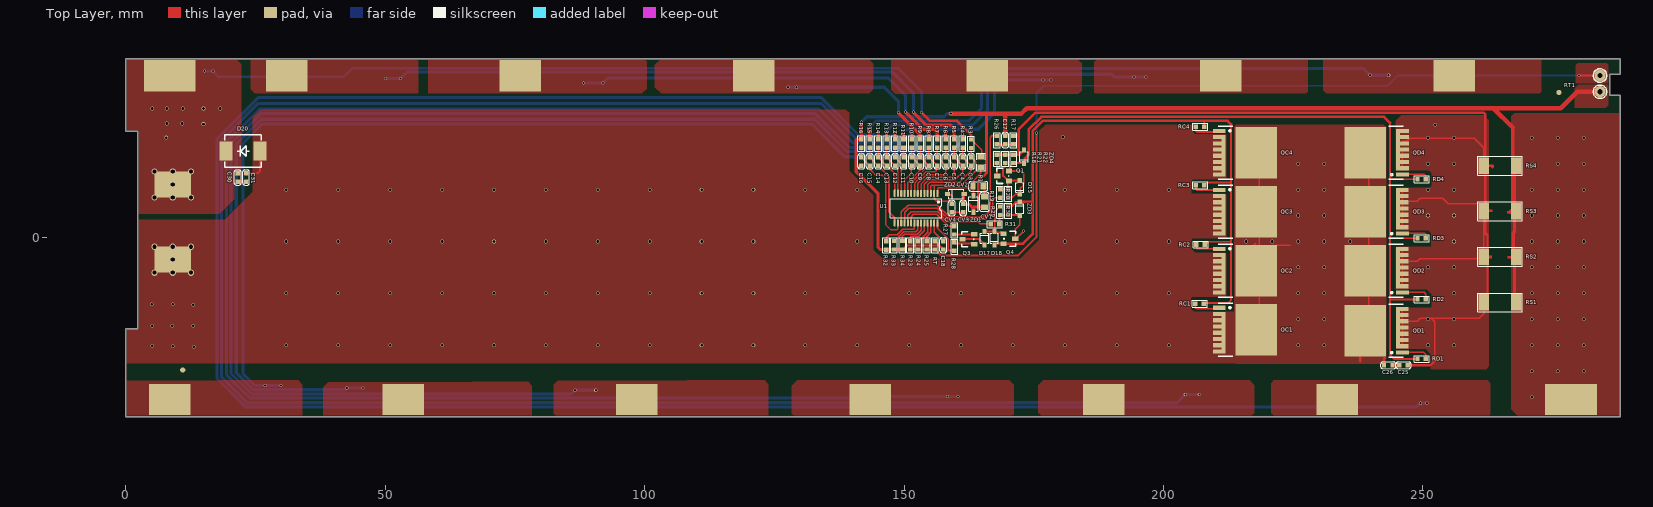
[diagram p0: Top Layer view]
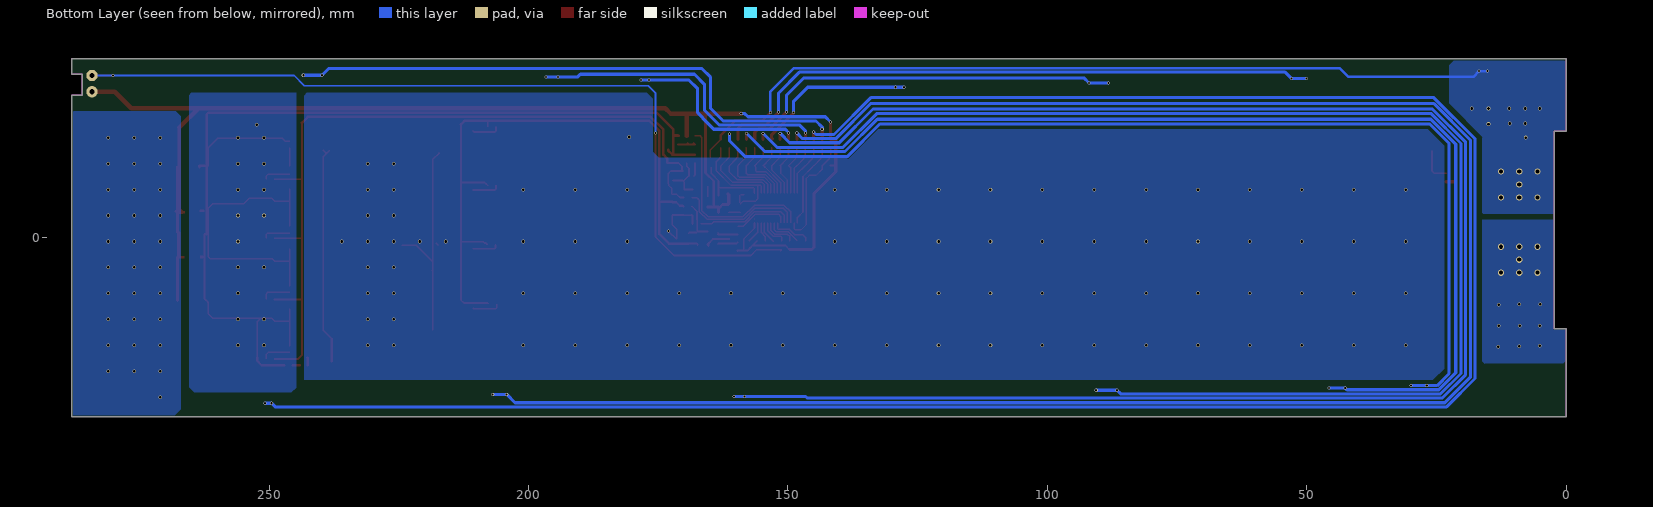
[diagram p1: Bottom Layer view, seen from below]
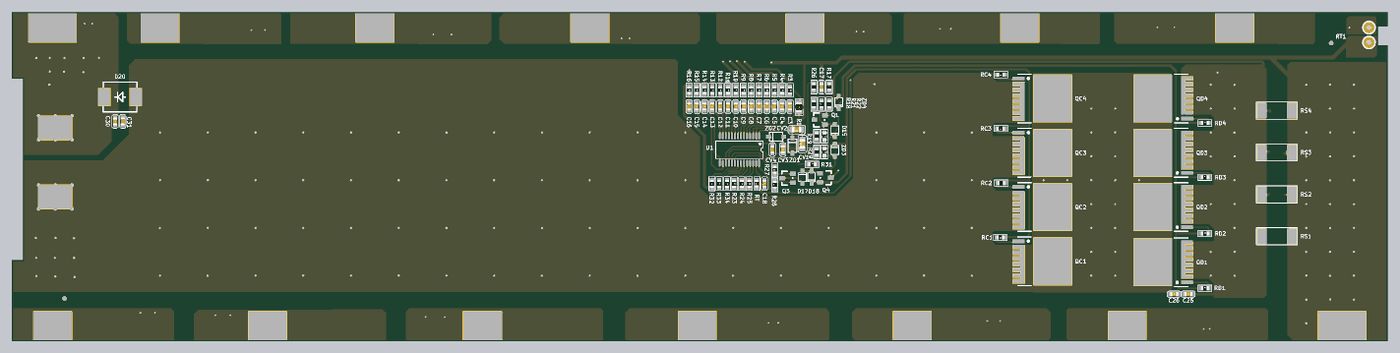
[diagram p2: 3D render of the assembled board from above, using the file's embedded part models]
# Altium PCB MISC84297.PcbDoc
Units mm, origin at the board's own origin, x right, y up, seen from the top; angles counter-clockwise.
Board outline 288 x 69 mm, 2 copper layers (Top Layer, Bottom Layer); 91 components, 64 nets, 295 pads, 210 vias.

## Layer stack, top to bottom (the 12.6 mil dielectric is the usual default, probably not edited)
Top Solder: solder mask 0.0102, Solder Resist, Dk 3.5
Top Layer: signal copper 0.0356
Dielectric 1: dielectric 0.32, FR-4, Dk 4.8
Bottom Layer: signal copper 0.0356
Bottom Solder: solder mask 0.0102, Solder Resist, Dk 3.5

## Board outline
0,-34.5 0,-17.5 2.3,-17.5 2.3,20.5 0,20.5 0,34.5 288,34.5 288,31.5 286,31.5 286,27.5 288,27.5 288,-34.5

## Design rules (kind name [scope] priority, off if disabled: settings)
Clearance [All] p1: gap=0.2 ignorepadtopadclearanceinfootprint=FALSE
ComponentClearance [All] p1: gap=0.2 collisioncheckmode=3 verticalgap=0.254 showdistances=FALSE
PolygonConnect [All] p1: connectstyle=Direct reliefconductorwidth=0.254 reliefentries=4 polygonreliefangle="90 Angle" airgapwidth=0.254
RoutingVias [All] p1: holewidth=0.4 width=0.6 viastyle="Through Hole" minholewidth=0.4 minwidth=0.6 maxholewidth=0.4 maxwidth=0.6
SolderMaskExpansion [All] p1: expansion=0.102 istentingtop=FALSE
SupplyNets "Schematic Supply Nets" [InNet('B-')] p1: voltage=0.000
Width [All] p1: maxlimit=1 minlimit=0.2 preferedwidth=0.25
29 further rules are at their usual default settings.

## Components (designator, comment, footprint, x,y, rotation, side; value= is the part's Value field where it differs from the comment)
C3 "104" CAP0603 162.922,14.7 r0 top
C4 "104" CAP0603 161.295,14.7 r0 top
C5 "104" CAP0603 159.668,14.7 r0 top
C6 "104" CAP0603 158.04,14.7 r0 top
C7 "104" CAP0603 156.413,14.7 r0 top
C8 "104" CAP0603 154.786,14.7 r0 top
C9 "104" CAP0603 153.158,14.7 r0 top
C10 "104" CAP0603 151.531,14.7 r0 top
C11 "104" CAP0603 149.904,14.7 r0 top
C12 "104" CAP0603 148.276,14.7 r0 top
C13 "104" CAP0603 146.649,14.7 r0 top
C14 "104" CAP0603 145.022,14.7 r0 top
C15 "104" CAP0603 143.395,14.7 r0 top
C16 "0.47uF" CAP0603 141.767,14.7 r0 top
C17 "104" CAP0603 169.5,18.8 r180 top
C18 "104" CAP0603 157.55,-1.467 r0 top
C25 "0.1uF" CAP0603 246.255,-24.587 r270 top
C26 "0.1uF" CAP0603 243.32,-24.587 r270 top
C30 "0.1uF" CAP0603 21.6,11.6 r180 top
C31 "0.1uF" CAP0603 23.2,11.6 r0 top
CV1 "2.2uF" CAP0805 165.5,6.9 r90 top
CV2 "2.2uF" CAP0805 164.3,9.9 r180 top
CV3 "0.1uF" CAP0603 161.4,5.7 r0 top
CV4 "0.1uF" CAP0603 159.2,5.7 r180 top
D15 "1N4148" SOD323 172.3,9.7 r270 top
D17 "1N4148" SOD323 165.5,-0.1 r90 top
D18 "1N4148" SOD323 167.4,-0.1 r270 top
D20 "RS3M" SMC 22.625,16.7 r180 top
Q1 "MMBT5401" SOT-23-3 169.1,11.9 r90 top
Q3 "MMBT5401" SOT-23-3 162.4,-0.3 r90 top
Q4 "MMBT5401" SOT-23-3 170.3,-0.2 r270 top
QC1 "NMOS" TOLL_123 214.383,-17.712 r270 top
QC2 "NMOS" TOLL_123 214.383,-6.349 r270 top
QC3 "NMOS" TOLL_123 214.383,5.021 r270 top
QC4 "NMOS" TOLL_123 214.383,16.388 r270 top
QD1 "NMOS" TOLL_123 242.393,-17.912 r90 top
QD2 "NMOS" TOLL_123 242.393,-6.349 r90 top
QD3 "NMOS" TOLL_123 242.393,5.021 r90 top
QD4 "NMOS" TOLL_123 242.422,16.388 r90 top
R1 "2K" RES0805 164.8,15.6 r270 top
R3 "2K" RES0603 162.922,18.1 r0 top
R4 "2K" RES0603 161.277,18.15 r0 top
R5 "2K" RES0603 159.651,18.15 r0 top
R6 "2K" RES0603 158.025,18.15 r0 top
R7 "2K" RES0603 156.399,18.15 r0 top
R8 "2K" RES0603 154.774,18.15 r0 top
R9 "2K" RES0603 153.148,18.15 r0 top
R10 "2K" RES0603 151.522,18.15 r0 top
R11 "2K" RES0603 149.896,18.15 r0 top
R12 "2K" RES0603 148.27,18.15 r0 top
R13 "2K" RES0603 146.645,18.15 r0 top
R14 "2K" RES0603 145.019,18.15 r0 top
R15 "2K" RES0603 143.393,18.15 r0 top
R16 "2K" RES0603 141.767,18.15 r0 top
R17 "1K" RES0603 171.1,18.8 r180 top
R18 "510R" RES0603 167.9,15.19 r180 top
R19 "1K" RES0603 168.5,8.5 r180 top
R20 "NC" RES0603 170.1,8.5 r0 top
R21 "5.1M" RES0603 169.5,15.2 r180 top
R22 "5.1M" RES0603 171.1,15.2 r180 top
R23 "270K" RES0603 151.185,-1.467 r0 top
R24 "41.2K" RES0603 152.776,-1.467 r0 top
R25 "22K" RES0603 154.367,-1.467 r0 top
R26 "10K" RES0603 167.9,18.8 r180 top
R27 "10K" RES0603 159.7,1.41 r180 top
R28 "3M" RES0603 159.7,-1.7 r180 top
R29 "5.1M" RES0603 168.5,5.2 r0 top
R30 "5.1M" RES0603 170.1,5.2 r0 top
R31 "1M" RES0603 167.51,2.6 r90 top
R32 "200K" RES0603 146.55,-1.482 r0 top
R33 "200K" RES0603 148.075,-1.457 r0 top
R34 "499K" RES0603 149.7,-1.457 r0 top
RC1 "47R" RES0603 206.955,-12.712 r270 top
RC2 "47R" RES0603 207.145,-1.312 r270 top
RC3 "47R" RES0603 207.045,10.088 r270 top
RC4 "47R" RES0603 207.055,21.388 r270 top
RD1 "47R" RES0603 249.745,-23.362 r90 top
RD2 "47R" RES0603 249.745,-11.887 r90 top
RD3 "47R" RES0603 249.745,-0.112 r90 top
RD4 "47R" RES0603 249.745,11.263 r90 top
RS1 "" 2512 264.795,-12.462 r90 top
RS2 "" 2512 264.795,-3.687 r90 top
RS3 "" 2512 264.795,5.088 r90 top
RS4 "" 2512 264.795,13.863 r90 top
RT "NC" RES0603 155.959,-1.467 r180 top
RT1 "103AT B=3435" WK 284.092,29.627 r270 top locked
U1 "CW1143" SSOP-28-0.635 152.322,5.7 r270 top locked
ZD1 "68V" SOD123 163.4,6.5 r90 top
ZD2 "68V" SOD123 160,8.4 r180 top
ZD3 "15V" SOD323 172.3,5.6 r90 top
ZD4 "15V" SOD323 173.1,15.6 r270 top

## Footprints (in the part's own frame and the unit in brackets; to place one, negate y for a bottom-side part, rotate by r counter-clockwise, add the part's x,y. Pads: shape width x height; smd on the part's side, far side on the other; paste and mask are expansions set on the pad)
2512 [mm]
  rect 3.2x2 smd: 1(0,3.05) 2(0,-3.15)
  silkscreen extent -1.8,-4.33 1.8,4.25
CAP0603 [mm] "CAP0402"
  rect 0.88x0.83 smd mask+0: 1(0,0.81) 2(0,-0.81)
  silkscreen extent -0.65,-1.45 0.65,1.45, body extent -0.41,-0.79 0.4,0.81, height 0.88
CAP0805 [mil]
  rect 43.31x50 smd: 1(-40,0)
  rect 40x50 smd: 2(40,0)
  silkscreen extent -73,-36 71,36, body extent -39,-25 39,25, height 35
RES0603 [mm] "CAP0402"
  rect 0.88x0.83 smd mask+0: 1(0,0.81) 2(0,-0.81)
  silkscreen extent -0.65,-1.45 0.65,1.45, body extent -0.4,-0.83 0.4,0.77, height 0.3
RES0805 [mil]
  rect 40x50 smd: 1(0,0) 2(80,0)
  silkscreen extent -28,-32 107,32, body extent 1,-25 79,24, height 4
SMC [mm]
  rect 2.44x3.62 smd: 1(-3.275,0) 2(3.275,0)
  silkscreen extent -3.55,-3.1 3.55,3.1
SOD123 [mm]
  rect 1x0.8 smd: 1(-1.6,0) 2(1.6,0)
  silkscreen extent -1.4,-0.9 1.4,0.9
SOD323 [mm]
  rect 1x0.8 smd: 1(-1.3,0) 2(1.3,0)
  silkscreen extent -0.92,-0.8 0.93,0.8
SOT-23-3 [mil]
  rect 36x47.24 smd: 1(-37.5,-43.94) 2(37.5,-43.94) 3(0.5,43.94)
  silkscreen extent -58,-41 58,49
SSOP-28-0.635 [mm]
  rect 1.4x0.4 smd: 1(-2.838,4.127) 28(2.862,4.128)
  oval 1.4x0.4 smd: 2(-2.838,3.492) 3(-2.838,2.857) 4(-2.838,2.222) 5(-2.838,1.587) 6(-2.838,0.952) 7(-2.838,0.317) 8(-2.838,-0.318) 9(-2.838,-0.953) 10(-2.838,-1.588) 11(-2.838,-2.223) 12(-2.838,-2.858) 13(-2.862,-3.493) 14(-2.862,-4.128) 15(2.862,-4.127) 16(2.862,-3.492) 17(2.862,-2.857) 18(2.862,-2.222) 19(2.862,-1.587) 20(2.862,-0.952) 21(2.862,-0.317) 22(2.862,0.318) 23(2.862,0.953) 24(2.862,1.588) 25(2.862,2.223) 26(2.862,2.858) 27(2.862,3.493)
  silkscreen extent -1.79,-4.96 1.86,4.96
TOLL_123 [mm] "贴片MOS"
  rect 0.8x2.5 smd: 1(-4.2,-3.638)
  rect 0.8x1.7 smd: 2(-3,-4) 2(-1.8,-4) 2(-0.6,-4) 2(0.6,-4) 2(1.8,-4) 2(3,-4) 2(4.2,-4)
  rect 8x0.8 smd: 2(0.6,-2.788)
  rect 9.9x8 smd: 3(0,3.5)
  silkscreen extent -5.1,-3.8 5.1,-1
WK [mm]
  round 2.2 hole 1: 1(-1.625,0.025) 2(1.5,0.025)
  silkscreen extent -2.91,-1.27 2.8,1.33

## Part data
C3 C4 C5 C6 C7 C8 C9 C10 C11 C12 C13 C14 C15 C16 C17 C18 C25 C26 C30 C31 CV1 CV2 CV3 CV4: library part CAP
D15 D17 D18 D20: library part DIODE, "DIODE"
Q1 Q3 Q4: library part PNP, "PNP Bipolar Transistor"
R1 R3 R4 R5 R6 R7 R8 R9 R10 R11 R12 R13 R14 R15 R16 R17 R18 R19 R20 R21 R22 R23 R24 R25 R26 R27 R28 R29 R30 R31 R32 R33 R34 RC1 RC2 RC3 RC4 RD1 RD2 RD3 RD4 RS1 RS2 RS3 RS4 RT: library part RES
RT1: library part RT1
ZD1 ZD2 ZD3 ZD4: library part "D Zener", "Zener Diode"

## Free pads (board coordinates)
  round 0.075 on Keep-Out: 1(-10.332,-6.165) 1(79.33,-42.487)
  rect 10x6 smd: 597(278.5,-31.2) 598(8.5,31.2)
  rect 7x5 smd: 598(9.075,-4.233) 598(9.075,10.267)
  rect 8x6 smd: 599(31,31.2) 600(8.5,-31.2) 601(53.5,-31.2) 602(76,31.2) 603(98.5,-31.2) 604(121,31.2) 605(143.5,-31.2) 606(166,31.2) 607(188.5,-31.2) 608(211,31.2) 609(233.5,-31.2) 610(256,31.2)
  round 1 smd: 649(276.2,28) 650(11,-25.5)

## Via types
v1: diameter 0.7, hole 0.5, Top Layer to Bottom Layer, tented both sides, 152 vias
v2: diameter 0.6, hole 0.4, Top Layer to Bottom Layer, tented both sides, 44 vias
v3: diameter 1.2, hole 0.8, Top Layer to Bottom Layer, tented both sides, 14 vias

## Nets (pads, with @x,y where several pads share a name; then routed paths per layer and width w, separated by ;. In a path a pad name is that pad's centre, name@x,y a point inside that pad or via, vN(x,y) a via of type N, cw(c..) or ccw(c..) an arc to the next point about the centre after c; other vN are vias at no path point)
B1: pad.610 R15.1 | length 111.1
  Top Layer w0.6: R15.1 143.393,20.893 v2(143.4,20.9)
  Bottom Layer w0.6: v2(143.4,20.9) 143.4,21.3 144.6,22.5 162.5,22.5 164.9,24.9 164.9,30.9 166.6,32.6 238.5,32.6 v2(239.8,31.3) v2(243.4,31.3)
B2: pad.609 R14.1 | length 417.4
  Top Layer w0.6: R14.1 145.1,19.041 v2(145.1,20.4)
  Bottom Layer w0.6: v2(145.1,20.4) 144.6,19.9 141.131,19.9 134.031,27 25.537,27 17.6,19.063 17.6,-27.131 23.069,-32.6 248.8,-32.6 v2(249.5,-31.9) v2(250.8,-31.9)
B3: pad.608 R13.1 | length 59.3
  Top Layer w0.6: R13.1 v2(146.645,20.155)
  Bottom Layer w0.6: v2(146.645,20.155) 146.645,20.645 147.7,21.7 163.2,21.7 166.1,24.6 166.1,29.6 168,31.5 190,31.5 190.5,31 v2(194.3,31) v2(196.6,31)
B4: pad.607 R12.1 | length 374.1
  Top Layer w0.6: R12.1 148.27,20.17 v2(148.3,20.2)
  Bottom Layer w0.6: v2(148.3,20.2) 147.2,19.1 140.8,19.1 134,25.9 25.569,25.9 18.5,18.831 18.5,-26.9 23.4,-31.8 202.6,-31.8 v2(204.2,-30.2) v2(206.9,-30.2)
B5: pad.606 R11.1 | length 36.7
  Top Layer w0.6: R11.1 149.896,20.196 v2(149.9,20.2)
  Bottom Layer w0.6: v2(149.9,20.2) 149.9,20.279 150.521,20.9 164.3,20.9 166.4,23 166.4,23.1 167.4,24.1 167.4,28.7 169.1,30.4 v2(176.8,30.4) v2(178.3,30.4)
B6: pad.605 R10.1 | length 327.1
  Top Layer w0.6: v2(151.5,20.1) 151.522,20.078 R10.1
  Bottom Layer w0.6: v2(151.5,20.1) 149.7,18.3 140.1,18.3 133.6,24.8 25.806,24.8 19.4,18.394 19.4,-26.394 23.906,-30.9 146.3,-30.9 146.6,-30.6 v2(158.4,-30.6) v2(160.413,-30.6)
B7: pad.604 R9.1 | length 31.7
  Top Layer w0.6: v2(148.9,24.1) 153.148,19.852 R9.1 153.033,19.075 R9.1@153.008,19.075
  Bottom Layer w0.6: v2(127.64,29) v2(129.3,29) 146.2,29 148.9,26.3 v2(148.9,24.1)
B8: pad.603 R8.1 | length 258.4
  Top Layer w0.6: R8.1 154.8,18.986 v2(154.8,20.1)
  Bottom Layer w0.6: v2(90.6,-29.4) v2(86.6,-29.4) 85.9,-30.1 24.237,-30.1 20.3,-26.163 20.3,18.163 26.037,23.9 132.9,23.9 139.4,17.4 152.1,17.4 v2(154.8,20.1)
B9: pad.602 R7.1 | length 76.2
  Top Layer w0.6: v2(150.3,24.2) 153.6,20.9 155.8,20.9 156.399,20.301 R7.1
  Bottom Layer w0.6: v2(88.2,29.8) v2(92,29.8) 93,30.8 146.9,30.8 150.3,27.4 v2(150.3,24.2)
B10: pad.601 R6.1 | length 213.8
  Top Layer w0.6: v2(158,20.1) 158.025,20.075 R6.1
  Bottom Layer w0.6: v2(45.7,-29) v2(42.6,-29) 42.3,-29.3 24.569,-29.3 21.3,-26.031 21.3,18.031 26.103,22.834 132.766,22.834 139,16.6 154.5,16.6 v2(158,20.1)
B11: pad.599 R5.1 | length 118.8
  Top Layer w0.6: v2(151.8,24.2) 154.3,21.7 159,21.7 159.651,21.049 R5.1
  Bottom Layer w0.6: v2(50.1,30.7) v2(53,30.7) 54.2,31.9 147.8,31.9 151.8,27.9 v2(151.8,24.2)
B12: pad.600 R4.1 | length 199.1
  Top Layer w0.6: R4.1 v2(161.277,19.977)
  Bottom Layer w0.6: v2(29.9,-28.5) v2(26.9,-28.5) 24.9,-28.5 22.6,-26.2 22.6,18.2 26.3,21.9 132.3,21.9 138.6,15.6 158.222,15.6 161.277,18.655 v2(161.277,19.977)
B+: C30.2 D20.2 pad.598@8.5,31.2 pad.598@9.075,10.267 R1.1 R3.1 | length 161.5
  Top Layer w0.3: R3.1 162.947,18.91 164.975,16.882 R1.1@164.975,15.557
  Top Layer w0.5: v2(153.4,24.1) 155,22.5 160.2,22.5 162.918,19.782 162.918,19.029 R3.1@162.922,19.025
  Bottom Layer w0.5: v2(15.2,32.1) v2(16.8,32.1) 17.9,31 42,31 43.65,32.65 148.9,32.65 153.4,28.15 v2(153.4,24.1)
  other v1: 7.8,19.3 15,21.9 7.9,22 10.9,22 5.1,24.9 7.9,24.9 11,24.9 15,24.9 18.2,24.9
  other v3: 5.575,7.767 9.075,7.767 12.575,7.767 9.075,10.267 5.575,12.767 9.075,12.767 12.575,12.767
B-: C16.2 C17.2 C18.2 CV1.1 CV3.1 pad.597 R16.1 R28.1 R32.2 R33.2 R34.2 RS1.2 RS2.2 RS3.2 RS4.2 RT1.2 RT.2 U1.28 ZD1.1 ZD2.1 | length 274.8
  Top Layer w0.3: U1.28 156.45,1.8 158.5,-0.25 158.5,-2.41 158.444,-2.466
  Top Layer w0.35: R34.2 149.725,-2.267 150.505,-1.487 156.814,-1.487 156.9,-1.573
  Top Layer w0.4: 140.782,14.065 140.957,13.89 C16.2 ; RT.2@155.984,-0.657 156.814,-1.487 ; 156.9,-1.573 157.31,-1.983 157.31,-2.062 C18.2@157.525,-2.277 ; C18.2 157.739,-2.466 158.444,-2.466 159.656,-2.466 R28.1
  Top Layer w0.5: 164.3,5.884 164.3,10.9 165.885,12.485 165.885,23.815 165.8,23.9
  Top Layer w0.6: R16.1 140.782,18.96 140.782,14.065 140.782,12.718 145,8.5 145,-1.9 145.367,-2.267 R34.2 ; R16.1@141.767,19.075 141.767,22.267 v2(141.8,22.3) ; ZD2.1 161.5,8.4 161.4,8.3 CV3.1 161.515,6.395 162.605,6.395 163.4,5.6 ZD1.1 ; 163.4,5.884 164.3,5.884 CV1.1 ; 266.695,4.913 267.3,5.518 267.3,21.2 ; 266.845,4.913 267.77,4.913 RS3.2 RS3.2@267.407,5.625 ; RS2.2@267.4,-3.687 267.4,0.999 ; RS1.2@267.645,-12.087 RS2.2@267.645,-3.687 ; 267.645,0.999 RS3.2@267.645,5.088 ; RS3.2@267.645,5.625 267.645,13.563 RS4.2@267.72,13.638
  Top Layer w0.8: v2(158.995,23.905) 159,23.9 165.8,23.9 169.4,23.9 ; C17.2 169.5,23.8 169.4,23.9 ; 267.3,21.2 263.55,24.95 ; RT1.2 279.727,28.127 276.55,24.95 263.55,24.95 ; 169.4,23.9 172.6,23.9 173.65,24.95 263.55,24.95
  Bottom Layer w0.6: v2(141.8,22.3) 142.8,23.3 157.7,23.3 158.305,23.905 v2(158.995,23.905)
  other v1: 270.978,-30.724 270.978,-25.724 275.978,-25.724 280.978,-25.724 270.978,-20.724 275.978,-20.724 280.978,-20.724 270.978,-15.724 275.978,-15.724 280.978,-15.724 270.978,-10.724 275.978,-10.724 280.978,-10.724 270.978,-5.724 275.978,-5.724 280.978,-5.724 270.978,-0.724 275.978,-0.724 280.978,-0.724 270.978,4.276 275.978,4.276 280.978,4.276 270.978,9.276 275.978,9.276 280.978,9.276 270.978,14.276 275.978,14.276 280.978,14.276 270.978,19.276 275.978,19.276 280.978,19.276
CO: R27.2 U1.20 | length 10.7
  Top Layer w0.25: U1.20 151.37,4.07 151.8,4.5 156.307,4.5 158.587,2.22 R27.2
CS: R26.2 U1.17 | length 36.9
  Top Layer w0.25: U1.17 149.465,4.965 150.8,6.3 156.436,6.3 158.736,4 165.4,4 166.6,5.2 166.6,19.289 166.921,19.61 R26.2 R26.2@168,19.61
DCTL: R32.1 U1.21 | length 7.9
  Top Layer w0.25: R32.1 146.55,-0.032 147.182,0.6 148.7,0.6 149.15,1.05 149.177,1.05 149.727,1.6 151.858,1.6 152.005,1.746 U1.21
DO: R19.1 U1.18 | length 24.6
  Top Layer w0.25: U1.18 150.1,4.9 150.9,5.7 156.4,5.7 158.55,3.55 165.586,3.55 167.05,5.014 167.05,7.25 167.49,7.69 ; 167.59,7.69 R19.1
NetC17_1: C17.1 R17.1 R26.1 | length 4
  Top Layer w0.25: R26.1@167.925,17.99 R26.1@168.215,18.28 ; C17.1@169.185,18.28 C17.1@169.475,17.99
  Top Layer w0.4: R26.1 R26.1@167.925,17.99 ; R26.1@168.025,17.99 169.575,17.99 R17.1@171.2,17.99
NetC18_1: C18.1 U1.27 | length 4.2
  Top Layer w0.25: U1.27 155.815,1.053 157.525,-0.657 C18.1
NetC25_1: C25.1 QD1.2 QD2.2 QD3.2 QD4.2 R17.2 R18.2 R21.2 R22.2 RS1.1 RS2.1 RS3.1 RS4.1 ZD4.1 | length 262.1
  Top Layer w0.25: QD1.2@246.031,-20.912 QD1.2@246.031,-16.112 ; QD1.2@246.031,-13.712 QD1.2@246.031,-16.112 ; QD2.2@246.031,-9.349 QD2.2@246.031,-4.549 ; QD2.2@246.031,-2.149 QD2.2@246.031,-4.549 ; QD3.2@246.031,2.214 QD3.2@246.031,7.014 ; QD3.2@246.031,9.414 QD3.2@246.031,7.014 ; QD4.2@246.031,13.777 QD4.2@246.031,17.377 ; QD4.2@246.031,18.577 246.901,18.577 247.492,19.169 259.863,19.169 261.745,17.288 RS4.1 ; 252.295,-23 252.295,-16.237 251.578,-15.52 ; RS1.1 261.745,-14.612 260.837,-15.52 251.578,-15.52 ; QD1.2@246.031,-16.112 248.923,-16.112 249.515,-15.52 251.578,-15.52 ; QD2.2@246.031,-4.549 248.923,-4.549 249.515,-3.957 249.621,-4.062 261.37,-4.062 RS2.1 261.745,0.7 RS3.1 261.745,5.688 260.87,6.563 254.863,6.563 253.82,7.606 249.515,7.606 248.923,7.014 QD3.2@246.031,7.014
  Top Layer w0.4: RS1.1 262.4,-11.807 262.4,0.663 ; 261.745,0.7 261.782,0.663 ; RS4.1 262,13.863 263.161,13.863 263.395,13.628
  Top Layer w0.45: R18.2 167.905,16.005 R21.2@169.6,16.005 ; R21.2 R22.2
  Top Layer w0.5: R22.2 171.11,16 172.3,16 173.1,16.8 ZD4.1 ; R17.2 171.19,19.7 172.1,19.7 ; 172.1,16.293 172.1,19.7 ; C25.1 251.408,-24.587 252.295,-23.7 252.295,-23 ; 261.782,0.663 262.4,0.663 ; 262,0.663 262,5.088 262,13.863 262,23.807 261.707,24.1 175.35,24.1 172.1,20.85 172.1,19.7 ; 263.395,13.628 263.395,13.863
  other v1: 250.978,-20.724 255.978,-20.724 250.978,-15.724 255.978,-15.724 255.978,-10.724 250.978,-5.724 255.978,-5.724 255.978,-0.724 250.978,4.276 255.978,4.276 250.978,9.276 255.978,9.276 250.978,14.276 255.978,14.276 250.978,19.276 255.978,19.276 252.4,21.8
NetC25_2: C25.2 C26.1 | length 1.3
  Top Layer w0.5: C26.1 C25.2
NetC30_1: C30.1 C31.2 | length 1.6
  Top Layer w0.6: C30.1 C31.2
NetCV1_2: CV1.2 CV2.1 | length 2
  Top Layer w0.3: CV2.1@165.416,9.9 165.416,8 CV1.2
NetCV3_2: CV3.2 CV4.1 | length 2.2
  Top Layer w0.3: CV4.1 159.205,4.885 161.395,4.885 CV3.2
NetD15_1: D15.1 Q1.1 R19.2 R20.1 R21.1 | length 9.5
  Top Layer w0.35: R19.2@168.4,9.31 170,9.31 170,10.731 Q1.1 ; R21.1 169.49,14.38 169.49,13.75 169.1,13.361 169.1,11.921 170.073,10.948 Q1.1 ; D15.1@172.2,11 170.268,11 Q1.1
NetD15_2: D15.2 Q1.2 R20.2 R22.1 RD1.1 RD2.1 RD3.1 RD4.1 ZD4.2 | length 157.9
  Top Layer w0.3: 243.67,-11.912 243.695,-11.887 ; 243.67,11.288 243.695,11.263
  Top Layer w0.35: R20.2 170.17,7.76 170.86,7.76 171.48,8.38 172.28,8.38 D15.2 172.4,8.5 172.4,9.5 172.963,10.063 172.963,10.232 173.075,10.345 173.075,12.325 172.547,12.853 Q1.2 170.45,13.086 170.45,13.765 171.075,14.39 R22.1 ZD4.2@173.01,14.39 ; 243.67,22.13 243.67,11.288 243.67,-0.112 ; 243.695,-11.887 RD2.1 ; 243.695,11.263 RD4.1 ; RD1.1 244.37,-23.362 243.67,-22.662 243.67,-11.912 243.67,-0.112 ; RD3.1 243.67,-0.112
  Top Layer w0.4: ZD4.2 ZD4.2@173.3,14.5
  Top Layer w0.5: ZD4.2@173.3,14.5 173.3,15.3 174,16 174,20.84 176.46,23.3 242.5,23.3 243.67,22.13
NetD17_1: D17.1 Q3.3 | length 4.9
  Top Layer w0.4: Q3.3 164.5,-0.287 164.5,-0.3 165.5,-1.3 D17.1 ; D17.1@165.3,-1.587 D17.1@165.3,-1.4
NetD17_2: D17.2 D18.1 Q4.1 R29.1 | length 9.1
  Top Layer w0.35: D17.2 D18.1 ; R29.1 168.475,6.01 167.55,5.085 167.55,3.545 167.49,3.485 167.49,1.29 D18.1 ; Q4.1@169.184,0.853 169.036,1 167.6,1 D18.1
NetD18_2: D18.2 Q4.2 R30.1 RC1.1 RC2.1 RC3.1 RC4.1 ZD3.2 | length 124.2
  Top Layer w0.25: RC1.1@207.765,-12.812 RC1.1@207.765,-12.787 ; RC2.1@208.094,-1.248 208.245,-1.097 RC2.1@208.27,-1.097
  Top Layer w0.35: RC1.1 207.877,-12.6 212.423,-12.6 213.02,-12.003 213.02,-0.765 ; 207.8,22.5 207.865,22.435 RC4.1 ; RC3.1 207.855,10.113 208.095,10.353 208.198,10.353 208.48,10.635 213.02,10.635 ; RC2.1 207.955,-1.287 208.195,-1.047 208.423,-1.047 208.705,-0.765 213.02,-0.765 ; 213.02,21.838 213.02,-0.765
  Top Layer w0.4: D18.2 167.4,-1.3 167.6,-1.1 169.132,-1.1 Q4.2 ; R30.1 170.247,6.157 170.857,6.157 171.534,6.834 172.234,6.834 ZD3.2 ; 174.7,6.9 174.8,6.8
  Top Layer w0.5: Q4.2 172.947,-1.152 174.8,0.7 174.8,6.8 174.8,20.6 176.7,22.5 207.8,22.5 212.358,22.5 213.02,21.838 ; ZD3.2 174.7,6.9
NetQ1_3: Q1.3 R18.1 | length 2.5
  Top Layer w0.35: R18.1 167.9,12.097 Q1.3@168.084,11.913
NetQ3_1: Q3.1 R28.2 | length 4
  Top Layer w0.35: R28.2 159.929,-1.119 163.383,-1.119 Q3.1
NetQ3_2: Q3.2 R27.1 | length 3.8
  Top Layer w0.35: R27.1 159.726,0.626 Q3.2@163.49,0.626 ; Q3.2@163.49,0.926 Q3.2@163.516,0.953
NetQC1_1: QC1.1 RC1.2 | length 5.5
  Top Layer w0.25: RC1.2@206.145,-12.812 206.145,-13.554 206.291,-13.7 210.557,-13.7 QC1.1
NetQC2_1: QC2.1 RC2.2 | length 5
  Top Layer w0.35: RC2.2@206.335,-1.412 206.335,-1.962 206.518,-2.146 QC2.1@210.745,-2.146
NetQC3_1: QC3.1 RC3.2 | length 5.2
  Top Layer w0.35: RC3.2 206.235,9.438 206.452,9.221 QC3.1
NetQC4_1: QC4.1 RC4.2 | length 5.4
  Top Layer w0.35: RC4.2 206.245,20.605 206.45,20.4 210.557,20.4 QC4.1
NetQD1_1: QD1.1 RD1.2 | length 5.5
  Top Layer w0.3: QD1.1 250.167,-22.112 250.555,-22.5 RD1.2
NetQD2_1: QD2.1 RD2.2 | length 5.7
  Top Layer w0.25: QD2.1 250.249,-10.549 250.555,-10.855 RD2.2
NetQD3_1: QD3.1 RD3.2 | length 5.4
  Top Layer w0.25: RD3.2 250.555,0.645
  Top Layer w0.3: QD3.1 250.379,0.821 250.555,0.645
NetQD4_1: QD4.1 RD4.2 | length 5.3
  Top Layer w0.25: RD4.2 250.555,11.913
  Top Layer w0.3: QD4.1 250.28,12.188 250.555,11.913
NetR23_1: R23.1 U1.24 | length 5.5
  Top Layer w0.25: R23.1 151.185,0.104 151.331,0.25 152.85,0.25 153.91,1.31 U1.24
NetR23_2: R23.2 R24.2 R25.2 RT1.1 RT.1 | length 168.5
  Top Layer w0.25: R23.2 R23.2@151.21,-2.277 ; R23.2@151.5,-2.567 R23.2@151.21,-2.277 ; RT.1 R25.2 R24.2 R23.2@151.21,-2.277
  Top Layer w0.35: RT.1 155.984,-2.277 157.107,-3.4 172,-3.4 175.55,0.15 v2(175.55,20.2) ; v2(280.048,31.252) RT1.1
  Bottom Layer w0.35: v2(175.55,20.2) 175.55,27.95 176.9,29.3 243.2,29.3 245.152,31.252 RT1.1
NetR24_1: R24.1 U1.25 | length 4.2
  Top Layer w0.25: R24.1 152.801,-0.657 154.545,1.087 U1.25
NetR25_1: R25.1 U1.26 | length 3.8
  Top Layer w0.25: R25.1 154.367,0.21 155.18,1.023 U1.26
NetR33_1: R33.1 U1.22 | length 6.6
  Top Layer w0.25: R33.1@148.194,-0.57 148.194,-0.553 148.39,-0.357 148.407,-0.357 149.914,1.15 152.25,1.15 152.64,1.54 U1.22
NetR34_1: R34.1 U1.23 | length 6.4
  Top Layer w0.25: R34.1 149.7,0.3 150.1,0.7 152.5,0.7 153.275,1.475 U1.23
P-: C26.2 C31.1 D20.1 pad.598@9.075,-4.233 Q4.3 QC1.2 QC1.3 QC2.2 QC2.3 QC3.2 QC3.3 QC4.2 QC4.3 QD1.3 QD2.3 QD3.3 QD4.3 R29.2 R30.2 R31.2 ZD3.1 | length 106.3
  Top Layer w0.25: QD1.3@237.92,-19.458 239.544,-17.834 239.544,15.611 238.845,16.31 QD4.3@238.334,16.821
  Top Layer w0.35: C31.1 25.43,12.41 25.9,12.88 D20.1 ; R31.2@168.41,2.6 168.41,4.3 R29.2 168.545,4.345 R30.2@170.1,4.345 ; R30.2 172.21,4.39 ZD3.1 172.3,2.486 171.416,1.602 Q4.3 171.559,-0.213 172.952,1.181 172.952,1.252 v2(173,1.3) ; QC4.3@217.232,16.31 218.442,15.1 QC2.3@218.442,-4.624 ; QC2.3@217.41,-1.454 217.727,-1.137 217.795,-1.137 ; QC1.3@218.442,-17.756 QC2.3@218.442,-6.389 ; QC2.3@218.56,-6.271 QC2.3@218.442,-6.389 ; 224.41,-1.454 221.612,-1.454 QC2.3@218.442,-4.624 ; QD4.3@238.845,16.31 238.998,16.31 QD4.3@239.544,16.855 ; QC2.3@218.442,-6.389 QC2.3@218.442,-4.624
  Top Layer w0.5: 237.92,-23.837 QD1.3@237.92,-19.458 ; C26.2 242.51,-23.19 242.6,-23.1
  other v1: 13.1,-21 9.1,-20.9 5.1,-20.8 30.978,-20.724 40.978,-20.724 50.978,-20.724 60.978,-20.724 70.978,-20.724 80.978,-20.724 90.978,-20.724 100.978,-20.724 110.978,-20.724 120.978,-20.724 130.978,-20.724 140.978,-20.724 150.978,-20.724 160.978,-20.724 170.978,-20.724 180.978,-20.724 190.978,-20.724 200.978,-20.724 225.978,-20.724 230.978,-20.724 5.1,-17 9,-17 13,-17 225.978,-15.724 230.978,-15.724 13,-12.9 5,-12.8 9.1,-12.8 30.978,-10.724 40.978,-10.724 50.978,-10.724 60.978,-10.724 70.978,-10.724 80.978,-10.724 90.978,-10.724 100.978,-10.724 110.978,-10.724 120.978,-10.724 130.978,-10.724 140.978,-10.724 150.978,-10.724 160.978,-10.724 170.978,-10.724 180.978,-10.724 190.978,-10.724 200.978,-10.724 225.978,-10.724 230.978,-10.724 225.978,-5.724 230.978,-5.724 30.978,-0.724 40.978,-0.724 50.978,-0.724 60.978,-0.724 70.978,-0.724 80.978,-0.724 90.978,-0.724 100.978,-0.724 110.978,-0.724 120.978,-0.724 130.978,-0.724 140.978,-0.724 180.978,-0.724 190.978,-0.724 200.978,-0.724 215.978,-0.724 220.978,-0.724 225.978,-0.724 230.978,-0.724 235.978,-0.724 225.978,4.276 230.978,4.276 30.978,9.276 40.978,9.276 50.978,9.276 60.978,9.276 70.978,9.276 80.978,9.276 90.978,9.276 100.978,9.276 110.978,9.276 120.978,9.276 130.978,9.276 140.978,9.276 180.978,9.276 190.978,9.276 200.978,9.276 225.978,9.276 230.978,9.276 225.978,14.276 230.978,14.276 180.6,19.4
  other v3: 5.575,-6.733 9.075,-6.733 12.575,-6.733 9.075,-4.233 5.575,-1.733 9.075,-1.733 12.575,-1.733
VC0: C15.2 C16.1 R16.2 U1.16 | length 21.6
  Top Layer w0.3: R16.2 C16.1 141.792,15.51 142.057,15.245 142.057,15.202 143.37,13.89 C15.2 143.396,13.888 143.396,13.201 144.597,12 145.847,12 146.5,11.347 146.5,2.472 147.472,1.5 148.654,1.5 148.83,1.676 U1.16
VC1: C14.2 C15.1 R15.2 U1.15 | length 16.5
  Top Layer w0.3: C15.1 143.42,15.51 143.685,15.245 143.685,15.202 144.997,13.89 C14.2 145.047,13.89 145.312,13.625 145.312,13.6 147.097,11.815 147.097,4.95 148.195,3.852 U1.15 ; C15.1@143.394,15.511 R15.2
VC2: C13.2 C14.1 R14.2 U1.14 | length 10.1
  Top Layer w0.3: R14.2 145.02,17.339 145.02,15.512 C14.1 145.047,15.51 145.312,15.245 145.312,15.202 146.624,13.89 C13.2 146.674,13.89 148.195,12.369 U1.14
VC3: C12.2 C13.1 R13.2 U1.13 | length 9.7
  Top Layer w0.3: R13.2 146.647,17.338 146.647,15.512 C13.1 146.674,15.51 146.939,15.245 146.939,15.202 148.251,13.89 C12.2 148.301,13.89 148.83,13.362 U1.13
VC4: C11.2 C12.1 R12.2 U1.12 | length 9.7
  Top Layer w0.3: R12.2 148.273,17.337 148.273,15.513 C12.1 148.301,15.51 148.566,15.245 148.566,15.202 C11.2@149.879,13.89 ; U1.12 149.465,13.476 C11.2@149.879,13.89 ; C11.2 C11.2@149.879,13.89
VC5: C10.2 C11.1 R11.2 U1.11 | length 10.1
  Top Layer w0.3: R11.2 149.9,17.336 149.9,15.514 C11.1 149.929,15.51 150.194,15.245 150.194,15.202 151.506,13.89 C10.2 151.347,13.706 151.347,12.375 150.1,11.127 U1.11
VC6: C9.2 C10.1 R10.2 U1.10 | length 10.5
  Top Layer w0.3: U1.10 150.735,10.652 153.108,13.025 153.108,13.84 C9.2 153.133,13.89 151.821,15.202 151.821,15.245 151.556,15.51 C10.1 151.527,15.515 151.527,17.336 R10.2
VC7: C8.2 C9.1 R9.2 U1.9 | length 11
  Top Layer w0.3: U1.9 151.37,10.58 154.415,13.625 154.521,13.625 C8.2 ; R9.2 153.153,17.335 153.153,15.515 C9.1 153.183,15.51 153.448,15.245 153.448,15.202 C8.2@154.761,13.89
VC8: C7.2 C8.1 R8.2 U1.8 | length 12.3
  Top Layer w0.3: U1.8@152.09,8.6 152.09,10.592 154.172,12.675 155.996,12.675 156.172,12.851 156.172,13.649 C7.2 156.388,13.89 156.123,14.155 156.123,14.198 154.811,15.51 C8.1 154.78,15.516 154.78,17.334 R8.2
VC9: C6.2 C7.1 R7.2 U1.7 | length 13.8
  Top Layer w0.3: U1.7 152.64,10.435 154.379,12.175 157.8,12.175 158.04,12.416 C6.2 158.015,13.89 157.75,14.155 157.75,14.198 156.438,15.51 C7.1 156.406,15.517 156.406,17.333 R7.2
VC10: C5.2 C6.1 R6.2 U1.6 | length 15
  Top Layer w0.3: U1.6 153.275,10.363 154.586,11.675 159.413,11.675 159.668,11.93 C5.2 159.643,13.89 159.378,14.155 159.378,14.198 158.065,15.51 C6.1 158.033,15.518 158.033,17.333 R6.2
VC11: C4.2 C5.1 R5.2 U1.5 | length 15.5
  Top Layer w0.3: U1.5 153.91,10.291 154.793,11.175 159.789,11.175 161.295,12.681 C4.2 161.27,13.89 159.958,15.202 159.958,15.245 159.693,15.51 C5.1 159.659,15.518 159.659,17.332 R5.2
VC12: C3.2 C4.1 R4.2 U1.4 | length 16.3
  Top Layer w0.3: U1.4 154.545,10.219 155.001,10.675 160.697,10.675 162.922,12.9 C3.2 162.897,13.89 162.632,14.155 162.632,14.198 161.32,15.51 C4.1 161.286,15.519 161.286,17.331 R4.2
VC13: C3.1 CV4.2 R3.2 U1.2 U1.3 ZD2.2 | length 24.9
  Top Layer w0.3: U1.3 155.18,9.974 155.355,10.15 155.847,10.15 ; ZD2.2 158.55,8.25 159.124,8.25 159.3,8.074 CV4.2@159.3,6.7 ; CV4.2@159.1,6.5 159.1,6.585 158.691,6.994 156.308,6.994 155.815,7.488 U1.2 155.815,10.118 155.847,10.15 ; R3.2 162.922,15.51 162.947,15.51 163.8,14.657 163.8,12.883 161.067,10.15 155.847,10.15
VDD: CV2.2 R1.2 U1.1 ZD1.2 | length 14.1
  Top Layer w0.3: U1.1 156.459,8.547 156.459,9.465 156.644,9.65 163.134,9.65 163.384,9.9 163.384,10.984 164.8,12.4 R1.2
  Top Layer w0.4: CV2.2@163.384,9.9 163.392,9.892 163.392,8.108 ZD1.2
VM: R31.1 U1.19 | length 18.8
  Top Layer w0.25: U1.19 150.735,4.3 151.435,5 156.464,5 158.364,3.1 164.3,3.1 164.7,2.7 166.69,2.7 R31.1@166.79,2.6

## Polygon pours and split planes (outlines as drawn)
B- on Top Layer "B-_L01_P088" (solid, pour order 88): 267,-15.2 267,-33.1 268.4,-34.5 288,-34.5 288,24 267.6,24 267,23.4
NetR23_2 on Top Layer "NETR23_2_L01_P093" (solid, remove dead copper, pour order 93): 285.5,29.8 285.7,30 285.7,33.3 285.4,33.6 279.8,33.6 279.4,33.2 279.4,29.8
B- on Top Layer "B-_L01_P092" (solid, pour order 92): 285.745,29.355 285.745,25.545 285.2,25 279.3,25 279.3,28.9 279.9,29.5 285.6,29.5
P- on Top Layer "NONET_L-01_P-001" (solid, remove dead copper, pour order 42): 144.1,-2.3 145.9,-4.1 172.4,-4.1 176.1,-0.4 176.1,20.6 177.3,21.8 205.4,21.8 205.6,21.6 205.6,20.4 206.1,19.9 212,19.9 212.063,19.837 212.063,11.238 205.763,11.238 205.363,10.837 205.363,8.612 205.475,8.5 211.914,8.5 212.113,8.301 212.113,-0.138 205.625,-0.138 205.363,-0.4 205.363,-2.163 206.113,-2.912 211.956,-2.912 212.113,-3.069 212.113,-11.412 205.563,-11.412 205.288,-11.688 205.288,-13.688 205.912,-14.312 211.993,-14.312 213.812,-14.312 218,-18.5 218.3,-18.5 218.3,-24.2 0,-24.2 0,2.3 1.2,3.5 19.1,3.5 24.5,8.9 24.5,23.3 25.9,24.7 138.8,24.7 139.4,24.1 139.4,12.9 144.1,8.2
B6 on Top Layer "NONET_L-01_P-001" (solid, remove dead copper, pour order 84): 129.387,-27.513 128.4,-28.5 128.4,-33.9 128.888,-34.388 152.337,-34.388 152.35,-34.4 170.5,-34.4 170.55,-34.45 170.65,-34.45 171.1,-34 171.1,-28.3 170.3,-27.5 170.287,-27.513
B2 on Top Layer "NONET_L-01_P-001" (solid, remove dead copper, pour order 86): 242.8,-27.515 221.285,-27.515 220.8,-28 220.8,-33.8 221.388,-34.388 242.337,-34.388 242.35,-34.4 262.6,-34.4 263,-34 263,-28.013 262.5,-27.513 243.162,-27.513
B4 on Top Layer "NONET_L-01_P-001" (solid, remove dead copper, pour order 85): 176.787,-27.513 175.9,-28.4 175.9,-33.7 176.588,-34.388 197.337,-34.388 197.35,-34.4 216.9,-34.4 217.5,-33.8 217.5,-28.4 216.613,-27.513
B8 on Top Layer "NONET_L-01_P-001" (solid, remove dead copper, pour order 83): 105.902,-27.529 83.271,-27.529 82.5,-28.3 82.5,-33.9 82.988,-34.388 107.337,-34.388 107.35,-34.4 123.8,-34.4 123.8,-28.2 123.113,-27.513 108.162,-27.513
B12 on Top Layer "NONET_L-01_P-001" (solid, remove dead copper, pour order 82): 16.702,-27.523 0.277,-27.523 -0.1,-27.9 -0.1,-34.1 0.188,-34.388 17.337,-34.388 17.35,-34.4 34,-34.4 34,-28.3 33.3,-27.513 18.162,-27.513
B+ on Top Layer "B+_L01_P081" (solid, pour order 81): 2.3,4.6 2.2,4.7 2.2,20.4 2.3,20.5 0,20.5 0,34.5 21.2,34.5 22.3,33.4 22.3,12.2 22,11.9 20.9,11.9 20.9,7.4 18.1,4.6
B7 on Top Layer "NONET_L-01_P-001" (solid, remove dead copper, pour order 80): 103.188,27.812 102,29 102,33.3 103.264,34.564 114.1,34.564 114.1,34.565 130.762,34.687 142.913,34.687 144.1,33.5 144.1,28.6 143.3,27.8 129.95,27.8 129.937,27.812
B3 on Top Layer "NONET_L-01_P-001" (solid, remove dead copper, pour order 79): 186.888,27.812 186.7,28 186.7,33.9 187.4,34.6 187.436,34.564 204.1,34.564 204.1,34.565 220.762,34.687 227.8,34.687 227.8,28.1 227.5,27.8 219.95,27.8 219.937,27.812
B1 on Top Layer "NONET_L-01_P-001" (solid, remove dead copper, pour order 78): 231.388,27.812 230.8,28.4 230.8,34.4 230.7,34.5 230.764,34.564 249.1,34.564 249.1,34.565 265.762,34.687 272.8,34.687 272.8,28.1 272.5,27.8 264.95,27.8 264.937,27.812
B9 on Top Layer "NONET_L-01_P-001" (solid, remove dead copper, pour order 77): 99.5,27.8 100.4,28.7 100.4,34 99.713,34.687 85.762,34.687 69.1,34.565 58.6,34.565 58.288,34.268 58.288,27.812 84.937,27.812 84.95,27.8
B5 on Top Layer "NONET_L-01_P-001" (solid, remove dead copper, pour order 76): 183.612,27.712 184.2,28.3 184.2,33.6 183.213,34.587 175.562,34.587 158.9,34.465 155.235,34.465 155.2,34.429 147.871,34.429 147.8,34.5 147.5,34.2 147.5,28.5 148.288,27.712
B11 on Top Layer "NONET_L-01_P-001" (solid, remove dead copper, pour order 75): 56.4,27.8 56.4,34 55.713,34.687 40.762,34.687 24.1,34.565 24.1,34.564 24.1,28.6 24.9,27.812 39.937,27.812 39.95,27.8
B10 on Top Layer "NONET_L-01_P-001" (solid, remove dead copper, pour order 47): 78.1,-34.5 78.3,-34.3 78.3,-28.5 77.6,-27.8 66.925,-27.8 66.913,-27.812 39.088,-27.812 38.1,-28.8 38.1,-34.4 38.387,-34.687 43.738,-34.687 67.463,-34.512 67.475,-34.5
P- on Top Layer "NONET_L-01_P-001" (solid, remove dead copper, pour order 41): 241.93,-24.3 242.893,-23.338 242.893,21.309 242.922,21.338 242.459,21.8 214,21.8 213.6,21.4 213.6,-24 214,-24.3
NetC25_1 on Top Layer "NONET_L-01_P-001" (solid, remove dead copper, pour order 40): 251.075,13 251.65,12.425 251.65,10.05 251.275,9.675 245,9.675 244.825,9.5 244.825,1.5 244.9,1.425 251.037,1.425 251.6,0.863 251.6,-1.7 251.55,-1.75 244.975,-1.75 244.8,-1.925 244.8,-10.1 247.15,-10.1 247.275,-9.975 247.275,-9.949 250.736,-9.949 251.675,-10.888 251.675,-13.35 251.5,-13.525 245.075,-13.525 244.825,-13.775 244.825,-21.4 250.525,-21.4 251.55,-22.425 251.55,-25.35 262.15,-25.35 262.7,-24.8 262.7,22.6 261.725,23.575 245.8,23.575 244.8,22.575 244.8,13
P- on Bottom Layer "P-_L02_P095" (solid, pour order 95): 2.3,-17.3 2.3,3.5 16.2,3.5 16.2,-23.8 15.7,-24.3 15.6,-24.2 0.6,-24.2 -0.3,-23.3 -0.1,-23.1 -0.1,-17.5 2.1,-17.5
B+ on Bottom Layer "B+_L02_P094" (solid, pour order 94): 16,4.6 16.2,4.8 16.2,19.3 16.1,19.4 22.6,25.9 22.6,29.3 22.6,33.2 21.7,34.1 0.4,34.1 0,34.5 0,20.5 2.3,20.5 2.3,4.9 2.6,4.6
P- on Bottom Layer "P-_L02_P091" (solid, pour order 91): 26.7,20.9 23.5,17.7 23.5,-25.281 25.731,-27.4 243.2,-27.4 243.2,27.4 242.7,27.9 177.2,27.9 176.1,26.8 176.1,16.6 174.9,15.4 138.1,15.4 132.6,20.9
NetC25_1 on Bottom Layer "NONET_L-01_P-001" (solid, remove dead copper, pour order 90): 244.8,27.9 265,27.9 265.4,27.5 265.4,-28.8 264.4,-29.8 245.7,-29.8 244.8,-28.9
B- on Bottom Layer "B-_L02_P089" (solid, pour order 89): 267,-15.2 267,-33.1 268.4,-34.5 288,-34.5 288,24 287.6,24.4 268,24.4 267,23.4

## Keep-outs
Keep-Out Layer:
  lines w0.1: 0,-34.5 0,-17.5 2.3,-17.5 2.3,20.5 0,20.5 0,34.5 288,34.5 288,31.5 286,31.5 286,27.5 288,27.5 288,-34.5 230.6,-34.5 0,-34.5

## Other copper
Top Layer:
  region net B-: 267.145,5.138 266.245,5.138 266.245,4.688 267.145,4.688
  region net NetC25_1: 263.37,5.463 262.445,5.463 262.445,4.963 263.37,4.963
  region net NetC25_1: 263.345,-3.437 262.645,-3.437 262.645,-4.037 263.345,-4.037
  region net B-: 267.245,-3.537 266.27,-3.537 266.27,-3.962 267.245,-3.962
  rectangle net B-: 156.272,3.5 156.647,3.7

## Silkscreen, mask and mechanical layers (free items; w line width, h text height)
Mechanical 1:
  lines w0.013: -20.694,-4.233 12.575,-4.233 ; -18.315,10.267 12.575,10.267 ; 3.5,31.2 260,31.2 ; 4.5,-31.2 237.5,-31.2 301.423,-31.2 ; 8.5,-56.038 8.5,-28.2 ; 8.5,28.2 8.5,55.143 ; 9.075,-6.233 9.075,12.767 ; 31,28.2 31,55.079 ; 53.5,-52.889 53.5,-28.2 ; 76,28.2 76,54.181 ; 98.5,-47.893 98.5,-28.2 ; 121,28.2 121,51.634 ; 143.5,-49.879 143.5,-28.2 ; 166,28.2 166,50.591 ; 188.5,-48.628 188.5,-28.2 ; 211,28.2 211,56.326 ; 233.5,-45.957 233.5,-28.2 ; 256,28.2 256,46.942 ; 278.5,-42.454 278.5,-27.2 ; 278.5,-34.2 278.5,-7.257 ; 283.101,29.627 292.821,29.627 ; 284.092,27.809 284.092,31.446 ; 283.101,27.809 285.082,27.809 285.082,31.446 283.101,31.446 283.101,27.809
  lines w0.1: -9.6,-22.5 290.4,-22.5 ; -2.6,22.5 297.4,22.5
  text "B1" at 253.774,38.344 h3.3
  text "B9" at 72.799,37.455 h3.3
  text "B+" at 6.505,36.566 h3.3
  text "B11" at 28.095,36.566 h3.3
  text "B7" at 117.249,35.931 h3.3
  text "B5" at 162.588,35.931 h3.3
  text "B3" at 207.038,35.55 h3.3
  text "NTC" at 289.842,28.184 h3.3
  text "CO" at 185.65,-24.525 h2
  text "B6" at 141.125,-38.999 h3.3
  text "B2" at 232.184,-38.999 h3.3
  text "B-" at 277.142,-39.507 h3.3
  text "B12" at 4.473,-39.634 h3.3
  text "B10" at 49.939,-40.015 h3.3
  text "B8" at 96.04,-40.015 h3.3
  text "B4" at 185.321,-40.269 h3.3